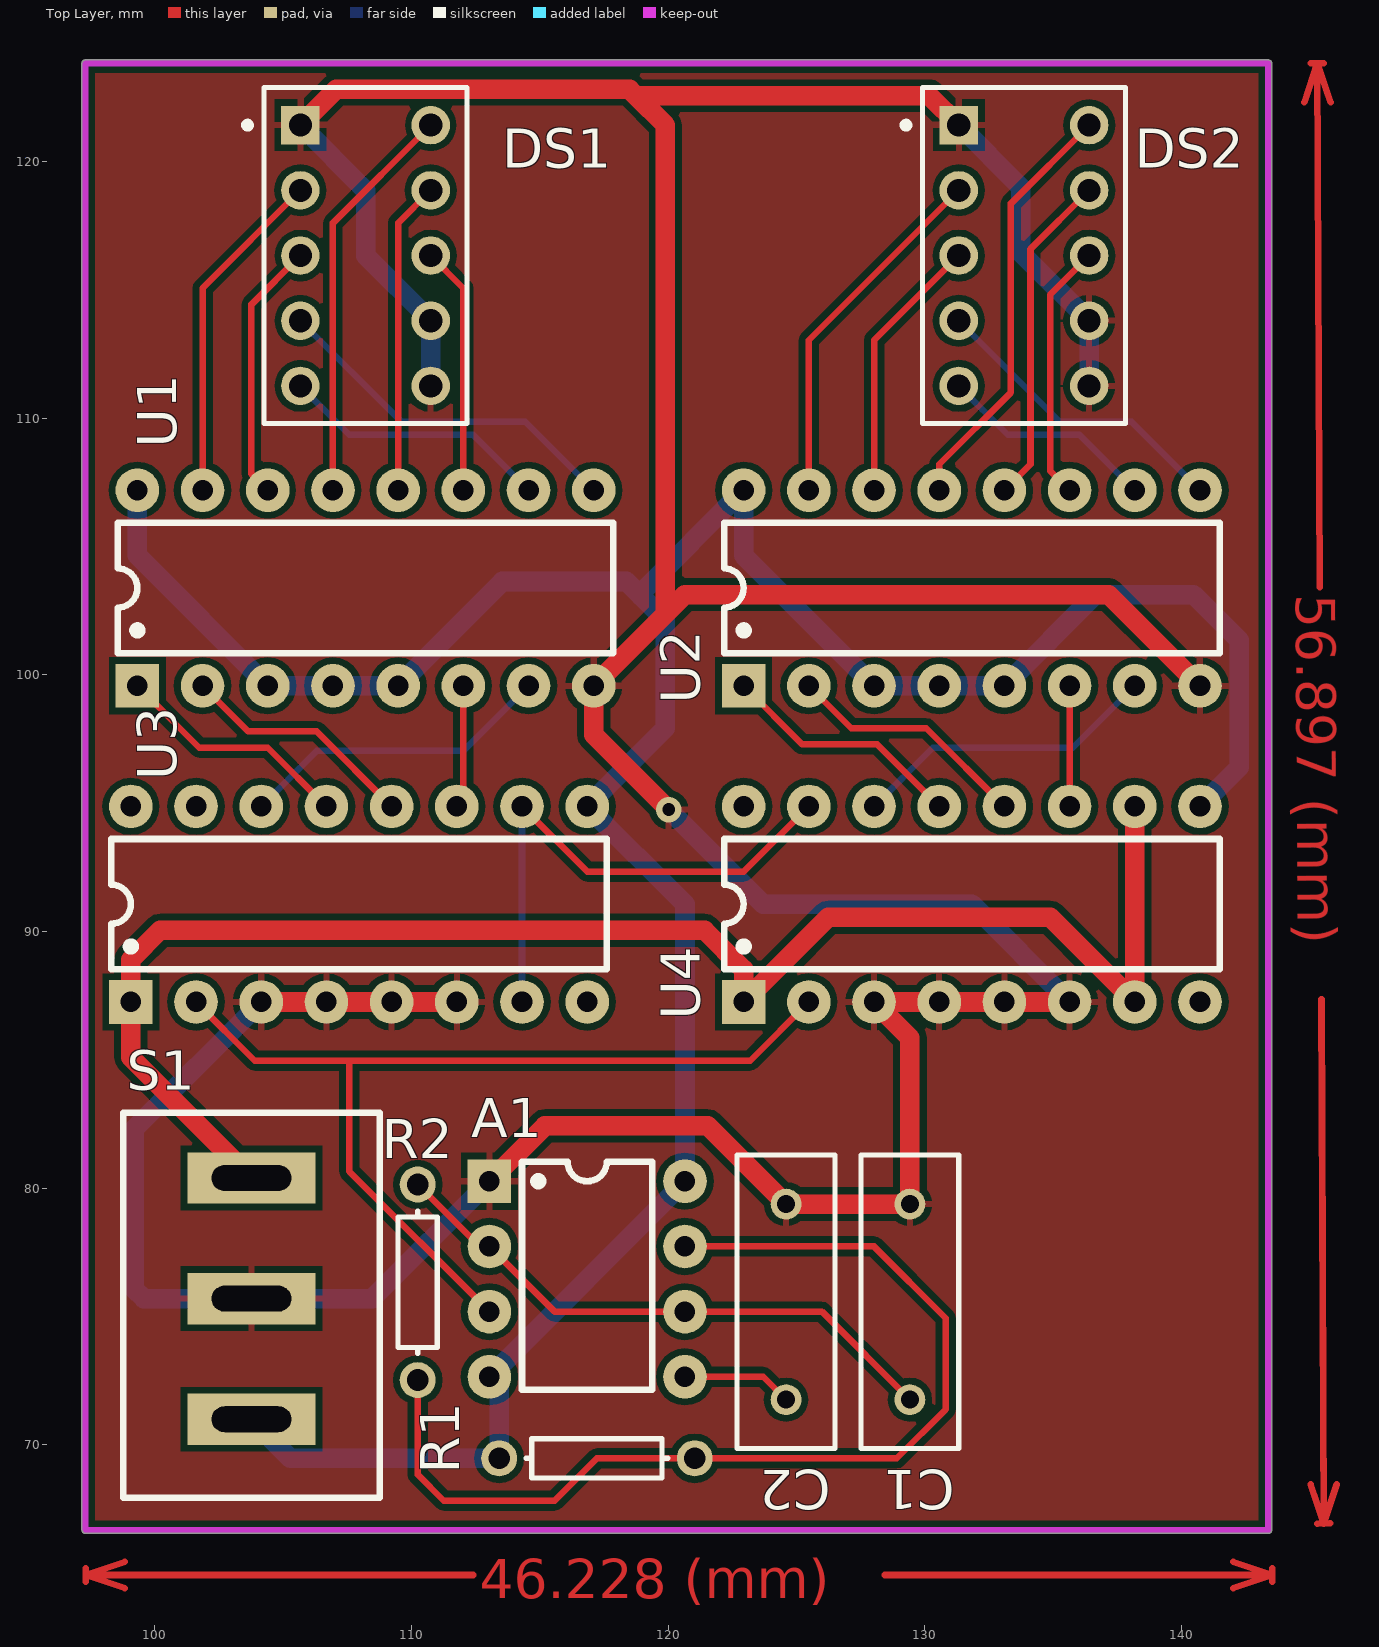
[diagram p0: Top Layer view]
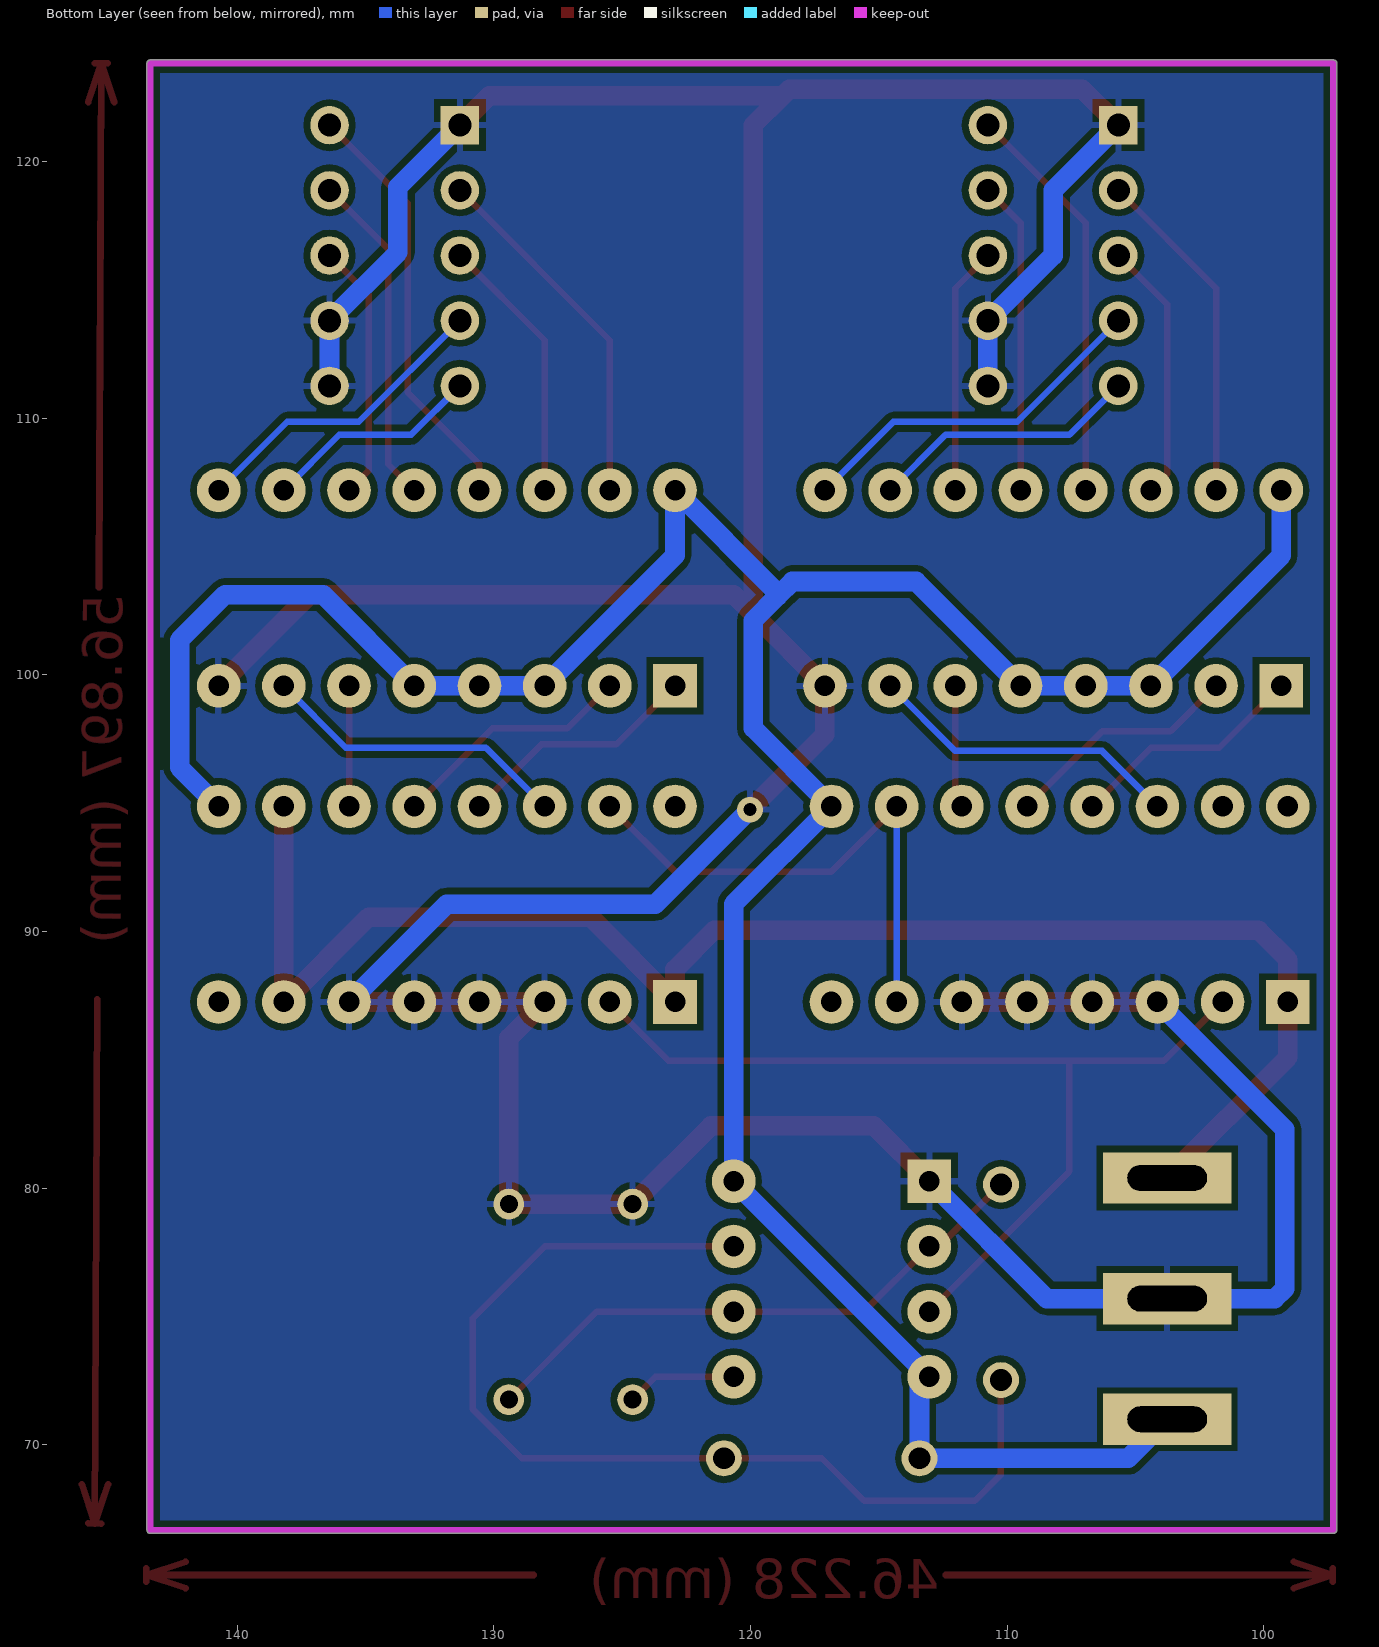
[diagram p1: Bottom Layer view, seen from below]
# Altium PCB MISC82818.PcbDoc
Units mm, origin at the board's own origin, x right, y up, seen from the top; angles counter-clockwise.
Board outline 46.36 x 57.4 mm, 2 copper layers (Top Layer, Bottom Layer); 12 components, 30 nets, 103 pads, 1 vias.

## Layer stack, top to bottom (the 12.6 mil dielectric is the usual default, probably not edited)
Top Solder: solder mask 0.0102, Solder Resist, Dk 3.5
Top Layer: signal copper 0.0356
Dielectric 1: dielectric 0.32, FR-4, Dk 4.8
Bottom Layer: signal copper 0.0356
Bottom Solder: solder mask 0.0102, Solder Resist, Dk 3.5

## Board outline
97.155,66.675 ccw(c97.282,66.675) 97.282,66.548 143.383,66.548 ccw(c143.383,66.675) 143.51,66.675 143.51,123.825 ccw(c143.383,123.825) 143.383,123.952 97.282,123.952 ccw(c97.282,123.825) 97.155,123.825

## Design rules (kind name [scope] priority, off if disabled: settings)
Clearance [All] p1: gap=0.254 ignorepadtopadclearanceinfootprint=FALSE except(0: Arc-Hole Track-Hole SMDPad-Hole THPad-Hole Via-Hole Fill-Hole Poly-Hole Region-Hole Text-Hole)
MinimumSolderMaskSliver [All] p1: minsoldermaskwidth=0
PolygonConnect [All] p1: connectstyle=Relief reliefconductorwidth=0.254 reliefentries=4 polygonreliefangle="90 Angle" airgapwidth=0.254
RoutingVias [All] p1: holewidth=0.711 width=1.27 viastyle="Through Hole" minholewidth=0.711 minwidth=1.27 maxholewidth=0.711 maxwidth=1.27
SilkToSilkClearance [All] p1: silktosilkclearance=0
SilkToSolderMaskClearance [IsPad] p1: minsilkscreentomaskgap=0 clearancetoexposedcopper=TRUE
SolderMaskExpansion [All] p1: expansion=0.102
Width [All] p1: maxlimit=0.762 minlimit=0.254 preferedwidth=0.254
27 further rules are at their usual default settings.

## Components (designator, comment, footprint, x,y, rotation, side; value= is the part's Value field where it differs from the comment)
A1 "555_VIRTUAL" DIP8 116.84,76.454 r0 top
C1 "3.3UF" RAD-0.3 129.413,75.565 r270 top
C2 "10NF" RAD-0.3 124.587,75.565 r270 top
DS1 "Dpy Green-CA" A 108.204,116.332 r0 top
DS2 "Dpy Green-CA" A 133.858,116.332 r0 top
R1 "10K" AXIAL-0.3 117.221,69.469 r180 top
R2 "10K" AXIAL-0.3 110.236,76.327 r270 top
S1 "SW-SPDT" SW-SPDT-3 103.759,75.441 r0 top
U1 "74LS48D" DIP16 108.204,103.378 r90 top
U2 "74LS48D" DIP16 131.826,103.378 r90 top
U3 "74LS160D" DIP16 107.95,91.059 r90 top
U4 "74LS160D" DIP16 131.826,91.059 r90 top

## Footprints (in the part's own frame and the unit in brackets; to place one, negate y for a bottom-side part, rotate by r counter-clockwise, add the part's x,y. Pads: shape width x height; smd on the part's side, far side on the other; paste and mask are expansions set on the pad)
A [mm] "LED, 7-Segment Display, 7.62 mm, RHD; 10 Leads; Row Space 5.08 mm; Pitch 2.54 mm"
  rect 1.5x1.5 hole 0.9: 1(-2.54,5.08)
  round 1.5 hole 0.9: 2(-2.54,2.54) 3(-2.54,0) 4(-2.54,-2.54) 5(-2.54,-5.08) 6(2.54,-5.08) 7(2.54,-2.54) 8(2.54,0) 9(2.54,2.54) 10(2.54,5.08)
  silkscreen extent -4.72,-6.55 3.95,6.55, body extent -3.95,-6.55 3.95,6.55, height 6.34
AXIAL-0.3 [mm] "Axial Device, Thru-Hole; 2 Leads; 0.3 in Pin Spacing"
  round 1.4 hole 0.85: 1(-3.81,0) 2(3.81,0)
  silkscreen extent -2.77,-0.76 2.77,0.76
DIP8 [mm]
  rect 1.7x1.7 hole 0.8: 1(-3.81,3.81)
  round 1.7 hole 0.8: 2(-3.81,1.27) 3(-3.81,-1.27) 4(-3.81,-3.81) 5(3.81,-3.81) 6(3.81,-1.27) 7(3.81,1.27) 8(3.81,3.81)
  silkscreen extent -2.54,-4.32 2.54,4.57, body extent -3.94,-4.7 3.91,4.7, height 4.5
DIP16 [mm]
  rect 1.7x1.7 hole 0.8: 1(-3.81,8.89)
  round 1.7 hole 0.8: 2(-3.81,6.35) 3(-3.81,3.81) 4(-3.81,1.27) 5(-3.81,-1.27) 6(-3.81,-3.81) 7(-3.81,-6.35) 8(-3.81,-8.89) 9(3.81,-8.89) 10(3.81,-6.35) 11(3.81,-3.81) 12(3.81,-1.27) 13(3.81,1.27) 14(3.81,3.81) 15(3.81,6.35) 16(3.81,8.89)
  silkscreen extent -2.54,-9.65 2.54,9.65, body extent -4.02,-9.65 4.02,9.65, height 4.45
RAD-0.3 [mm] "Radial Cap, Thru-Hole; 2 Leads; 0.3 in Pin Spacing"
  round 1.2 hole 0.7: 1(-3.81,0) 2(3.81,0)
  silkscreen extent -5.71,-1.91 5.71,1.91
SW-SPDT-3 [mm]
  rect 5x2 hole 1 slot 3.1 at 0 deg paste+0 mask+0.051: 1(0,0.25) 2(0,4.95) 3(0,-4.45)
  silkscreen extent -5,-7.5 5,7.5

## Part data
C1 C2: library part Cap, "Capacitor"
DS1 DS2: "7.62 mm Black Surface Green 7-Segment Display: CA, RH DP"
R1 R2: library part Res1, "Resistor"
S1: "SPDT Subminiature Toggle Switch, Right Angle Mounting, Vertical Actuation"
U1 U2: library part SN74LS48D, "BCD-to-Seven-Segment Decoder/Driver"

## Via types
v1: diameter 1, hole 0.5, Top Layer to Bottom Layer, 1 vias

## Nets (pads, with @x,y where several pads share a name; then routed paths per layer and width w, separated by ;. In a path a pad name is that pad's centre, name@x,y a point inside that pad or via, vN(x,y) a via of type N, cw(c..) or ccw(c..) an arc to the next point about the centre after c; other vN are vias at no path point)
+5: A1.4 A1.8 R1.2 S1.3 U1.3 U1.4 U1.5 U1.16 U2.3 U2.4 U2.5 U2.16 U3.9 U4.9 | length 115.7
  Bottom Layer w0.762: U1.16 99.314,104.648 U1.3 U1.4 U1.5 113.538,103.632 118.364,103.632 118.935,103.06 ; S1.3 105.281,69.469 R1.2 113.411,72.263 A1.4 A1.8 120.65,91.059 U3.9 119.888,97.917 119.888,102.108 118.935,103.06 ; U4.9 142.24,96.393 142.24,101.346 140.462,103.124 136.652,103.124 U2.5 U2.4 U2.3 122.936,104.648 U2.16 118.935,103.188 118.935,103.06
GND: A1.1 C1.1 C2.1 DS1.1 DS1.6 DS1.7 DS2.1 DS2.6 DS2.7 S1.1 U1.8 U2.8 U3.3 U3.4 U3.5 U3.6 U4.3 U4.4 U4.5 U4.6 | length 194.7
  Top Layer w0.762: U3.3 U3.4 U3.5 U3.6 ; DS1.1 107.061,122.809 118.491,122.809 118.745,122.555 ; A1.1 115.189,82.423 121.539,82.423 C2.1 C1.1 129.413,85.852 U4.3 U4.4 U4.5 U4.6 ; v1(120.015,94.742) 117.094,97.663 U1.8 119.888,102.362 ; DS2.1 130.175,122.555 118.745,122.555 ; U2.8 137.16,103.124 120.65,103.124 119.888,102.362 ; 118.745,122.555 119.888,121.412 119.888,102.362
  Bottom Layer w0.762: U3.3 99.187,82.296 99.187,76.073 99.569,75.691 S1.1 108.457,75.691 A1.1 ; DS1.1 108.204,118.872 108.204,116.332 DS1.7 DS1.6 ; v1(120.015,94.742) 123.698,91.059 131.826,91.059 U4.6 ; DS2.1 133.731,118.999 133.731,116.459 DS2.7 DS2.6
NetA1_2: A1.2 A1.6 C1.2 R2.1 | length 22.6
  Top Layer w0.254: R2.1 112.649,77.724 A1.2 115.57,75.184 A1.6 125.984,75.184 C1.2
NetA1_3: A1.3 U3.2 U4.2 | length 37.8
  Top Layer w0.254: U3.2 103.886,84.963 107.569,84.963 ; A1.3 107.569,80.645 107.569,84.963 ; U4.2 123.19,84.963 107.569,84.963
NetA1_5: A1.5 C2.2 | length 4.3
  Top Layer w0.254: A1.5 123.698,72.644 C2.2
NetA1_7: A1.7 R1.1 R2.2 | length 41
  Top Layer w0.254: R2.2 110.236,68.834 111.252,67.818 115.57,67.818 117.221,69.469 R1.1 128.905,69.469 130.81,71.374 130.81,74.93 128.016,77.724 A1.7
NetDS1_2: DS1.2 U1.15 | length 13.3
  Top Layer w0.254: U1.15 101.854,115.062 DS1.2
NetDS1_3: DS1.3 U1.14 | length 10.2
  Top Layer w0.254: U1.14 103.759,107.823 103.759,114.427 DS1.3
NetDS1_4: DS1.4 U1.9 | length 14.2
  Bottom Layer w0.254: DS1.4 109.601,109.855 114.427,109.855 U1.9
NetDS1_5: DS1.5 U1.10 | length 10.6
  Bottom Layer w0.254: DS1.5 107.569,109.347 112.395,109.347 U1.10
NetDS1_8: DS1.8 U1.11 | length 9.7
  Top Layer w0.254: DS1.8 112.014,115.062 U1.11
NetDS1_9: DS1.9 U1.12 | length 12.2
  Top Layer w0.254: U1.12 109.474,117.602 DS1.9
NetDS1_10: DS1.10 U1.13 | length 15.8
  Top Layer w0.254: U1.13 106.934,117.602 DS1.10
NetDS2_2: DS2.2 U2.15 | length 14.1
  Top Layer w0.254: U2.15 125.476,113.03 DS2.2
NetDS2_3: DS2.3 U2.14 | length 10.5
  Top Layer w0.254: U2.14 128.016,113.03 DS2.3
NetDS2_4: DS2.4 U2.9 | length 12.1
  Bottom Layer w0.254: DS2.4 135.255,109.855 138.049,109.855 U2.9
NetDS2_5: DS2.5 U2.10 | length 8.5
  Bottom Layer w0.254: DS2.5 133.223,109.347 136.017,109.347 U2.10
NetDS2_8: DS2.8 U2.11 | length 10.1
  Top Layer w0.254: U2.11 134.874,107.95 134.874,114.808 DS2.8
NetDS2_9: DS2.9 U2.12 | length 13.1
  Top Layer w0.254: U2.12 134.112,108.204 134.112,116.586 DS2.9
NetDS2_10: DS2.10 U2.13 | length 16.6
  Top Layer w0.254: U2.13 130.556,108.204 133.35,110.998 133.35,118.364 DS2.10
NetS1_2: S1.2 U3.1 U4.1 U4.7 U4.10 | length 62.3
  Top Layer w0.762: S1.2 99.06,85.09 U3.1 99.06,88.9 100.203,90.043 121.412,90.043 122.936,88.519 U4.1 126.238,90.551 134.874,90.551 U4.7 U4.10
NetU1_1: U1.1 U3.13 | length 9.3
  Top Layer w0.254: U1.1 101.727,97.155 104.394,97.155 U3.13
NetU1_2: U1.2 U3.12 | length 9.3
  Top Layer w0.254: U1.2 103.632,97.79 106.299,97.79 U3.12
NetU1_6: U1.6 U3.11 | length 4.8
  Top Layer w0.254: U3.11 112.014,95.123 U1.6
NetU1_7: U1.7 U3.14 | length 12.4
  Bottom Layer w0.254: U3.14 106.299,97.028 112.014,97.028 U1.7
NetU2_1: U2.1 U4.13 | length 9.6
  Top Layer w0.254: U2.1 125.222,97.282 128.143,97.282 U4.13
NetU2_2: U2.2 U4.12 | length 9.6
  Top Layer w0.254: U2.2 127.127,97.917 130.048,97.917 U4.12
NetU2_6: U2.6 U4.11 | length 4.7
  Top Layer w0.254: U4.11 U2.6
NetU2_7: U2.7 U4.14 | length 12.1
  Bottom Layer w0.254: U4.14 130.302,97.155 135.763,97.155 U2.7
NetU3_7: U3.7 U3.10 U4.15 | length 20.9
  Top Layer w0.254: U3.10 116.84,92.329 122.936,92.329 U4.15
  Bottom Layer w0.254: U3.7 U3.10
pads on no net: U3.8 U3.15 U3.16 U4.8 U4.16
copper on no net: | length 85.9
  Top Layer w0.254: 97.305,64.668 97.305,65.176 ; 98.829,64.414 97.305,64.922 ; 98.829,65.43 97.305,64.922 ; 112.395,64.922 97.305,64.922 ; 128.443,64.922 143.533,64.922 ; 142.009,64.414 143.533,64.922 ; 142.009,65.43 143.533,64.922 ; 143.533,64.668 143.533,65.176 ; 144.787,122.299 145.288,123.825 ; 145.027,68.451 145.542,66.929 ; 145.034,123.824 145.542,123.826 ; 145.288,66.928 145.796,66.93 ; 145.379,103.401 145.288,123.825 ; 145.451,87.353 145.542,66.929 ; 145.803,122.303 145.288,123.825 ; 146.043,68.455 145.542,66.929

## Polygon pours and split planes (outlines as drawn)
GND on Top Layer "Top Layer-No Net" (solid, remove dead copper, pour order 0): 86.487,128.016 88.011,129.54 161.29,129.54 161.29,73.152 144.272,56.134 74.803,56.134
GND on Bottom Layer "Top Layer-No Net" (solid, remove dead copper, pour order 2): 87.503,132.715 147.574,132.715 152.908,127.381 152.908,50.038 90.551,50.038 80.645,59.944

## Keep-outs
Keep-Out Layer:
  lines w0.254: 103.251,123.825 104.14,123.825 143.383,123.825 143.383,69.342 143.383,66.675 97.282,66.675 97.282,123.825 103.759,123.825

## Other copper
Top Layer:
  text "56.897 (mm)" at 144.466,103.143 h1.52 r270.26
  text "46.228 (mm)" at 112.649,64.008 h1.52